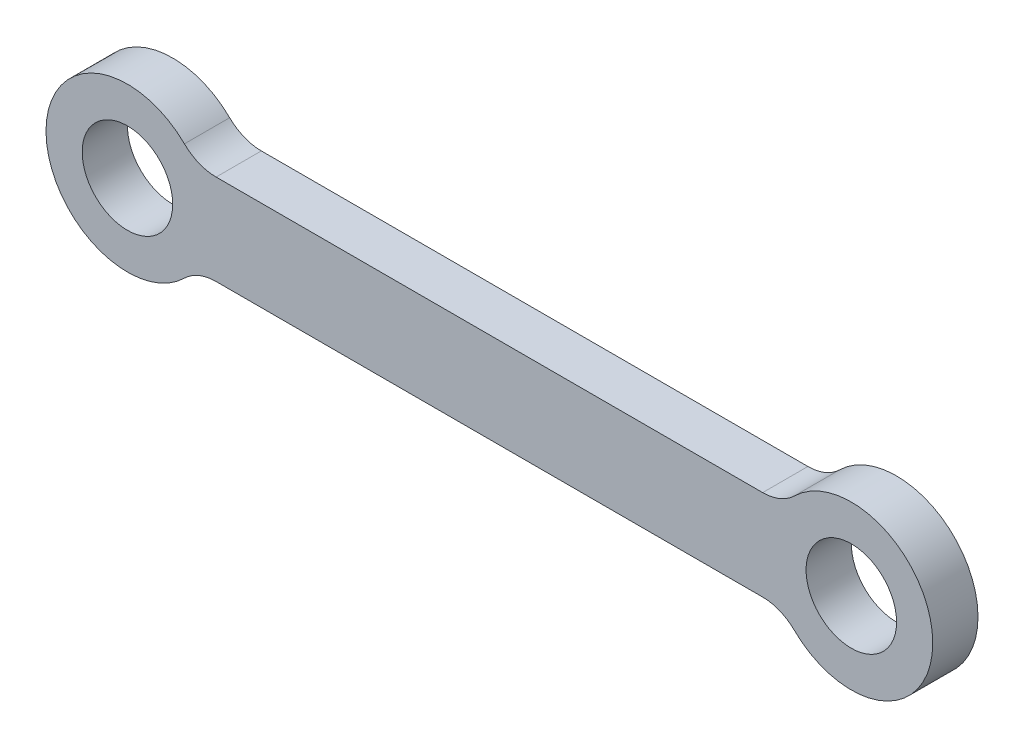
from build123d import *

# Parameters (mm, degrees)
SKETCH1_R           = 5
BOSS_EXTRUDE1_DEPTH = 5


with BuildPart() as part:
    # Sketch1 → Boss-Extrude1 (new body)
    with BuildSketch(Plane.XY):
        with BuildLine():
            Line((9.797958971, 5), (70.202041029, 5))
            ThreePointArc((70.202041029, 5), (72.091863394, 5.370899501), (73.70131209, 6.428571429))
            ThreePointArc((73.70131209, 6.428571429), (89, 0), (73.70131209, -6.428571429))
            ThreePointArc((73.70131209, -6.428571429), (72.091863394, -5.370899501), (70.202041029, -5))
            Line((70.202041029, -5), (9.797958971, -5))
            ThreePointArc((9.797958971, -5), (7.908136606, -5.370899501), (6.29868791, -6.428571429))
            ThreePointArc((6.29868791, -6.428571429), (-9, 0), (6.29868791, 6.428571429))
            ThreePointArc((6.29868791, 6.428571429), (7.908136606, 5.370899501), (9.797958971, 5))
        make_face()
        Circle(SKETCH1_R, mode=Mode.SUBTRACT)
        with Locations((80, 0)):
            Circle(SKETCH1_R, mode=Mode.SUBTRACT)
    extrude(amount=BOSS_EXTRUDE1_DEPTH)


solid = part.part
